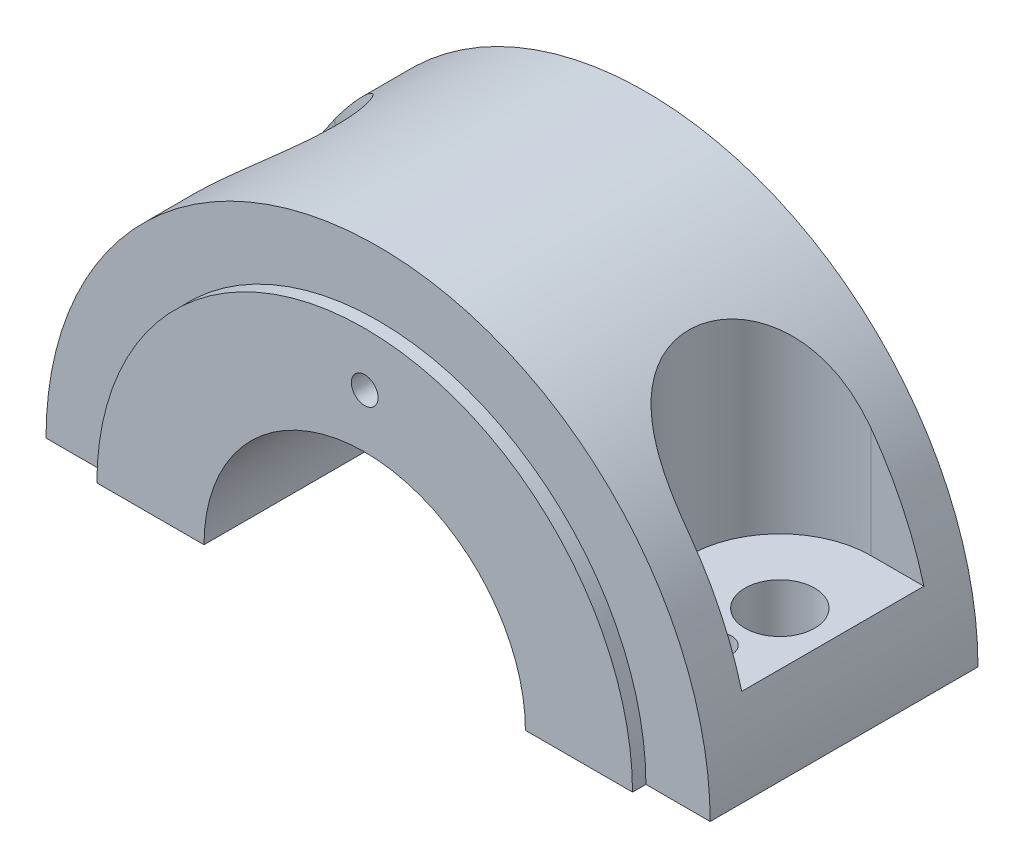
from build123d import *

# Parameters (mm, degrees)
BOSS_EXTRUDE1_DEPTH   = 25
BOSS_EXTRUDE2_DEPTH   = 27.5
CUT_EXTRUDE1_DEPTH    = 82.952730278
SKETCH4_R             = 6.5
SKETCH4_R_2           = 3
CUT_EXTRUDE2_DEPTH    = 82.95273041
M6_TAPPED_HOLE1_D     = 5
M6_TAPPED_HOLE1_DEPTH = 17
M6_TAPPED_HOLE1_TIP   = 1.502151548


with BuildPart() as part:
    # Sketch1 → Boss-Extrude1 (new, symmetric)
    with BuildSketch(Plane.XY):
        with BuildLine():
            Line((-62, 0), (-30, 0))
            ThreePointArc((-30, 0), (0, 30), (30, 0))
            Line((30, 0), (62, 0))
            ThreePointArc((62, 0), (0, 62), (-62, 0))
        make_face()
    extrude(amount=BOSS_EXTRUDE1_DEPTH, both=True)

    # Sketch2 → Boss-Extrude2 (add, symmetric)
    with BuildSketch(Plane.XY):
        with BuildLine():
            Line((-50, 0), (-30, 0))
            ThreePointArc((-30, 0), (0, 30), (30, 0))
            Line((30, 0), (50, 0))
            ThreePointArc((50, 0), (0, 50), (-50, 0))
        make_face()
    extrude(amount=BOSS_EXTRUDE2_DEPTH, both=True)

    # Sketch3 → Cut-Extrude1 (cut, through all)
    with BuildSketch(Plane(origin=(0, 16, 0), x_dir=(1, 0, 0), z_dir=(0, 1, 0))):
        with BuildLine():
            Line((-75, 17), (-50, 17))
            ThreePointArc((-50, 17), (-33, 0), (-50, -17))
            Line((-50, -17), (-75, -17))
            Line((-75, -17), (-75, 17))
        make_face()
        with BuildLine():
            Line((75, -17), (50, -17))
            ThreePointArc((50, -17), (33, 0), (50, 17))
            Line((50, 17), (75, 17))
            Line((75, 17), (75, -17))
        make_face()
    extrude(amount=CUT_EXTRUDE1_DEPTH, mode=Mode.SUBTRACT)

    # Sketch4 → Cut-Extrude2 (cut, through all)
    with BuildSketch(Plane(origin=(0, 16, 0), x_dir=(1, 0, 0), z_dir=(0, 1, 0))):
        with Locations(Location((-50, 0, 0), (0, 0, 270))):
            Circle(SKETCH4_R)
        with Locations(Location((-50, 12, 0), (0, 0, 270))):
            Circle(SKETCH4_R_2)
        with Locations(Location((50, 0, 0), (0, 0, 90))):
            Circle(SKETCH4_R)
        with Locations(Location((50, -12, 0), (0, 0, 270))):
            Circle(SKETCH4_R_2)
    extrude(amount=-CUT_EXTRUDE2_DEPTH, mode=Mode.SUBTRACT)

    # M6 Tapped Hole1
    with Locations(Plane.XY.offset(27.5)):
        with Locations((0, 40)):
            Hole(M6_TAPPED_HOLE1_D / 2, depth=M6_TAPPED_HOLE1_DEPTH)
            with Locations((0, 0, -(M6_TAPPED_HOLE1_DEPTH + M6_TAPPED_HOLE1_TIP / 2))):  # 118° drill point
                Cone(0, M6_TAPPED_HOLE1_D / 2, M6_TAPPED_HOLE1_TIP, mode=Mode.SUBTRACT)


solid = part.part
